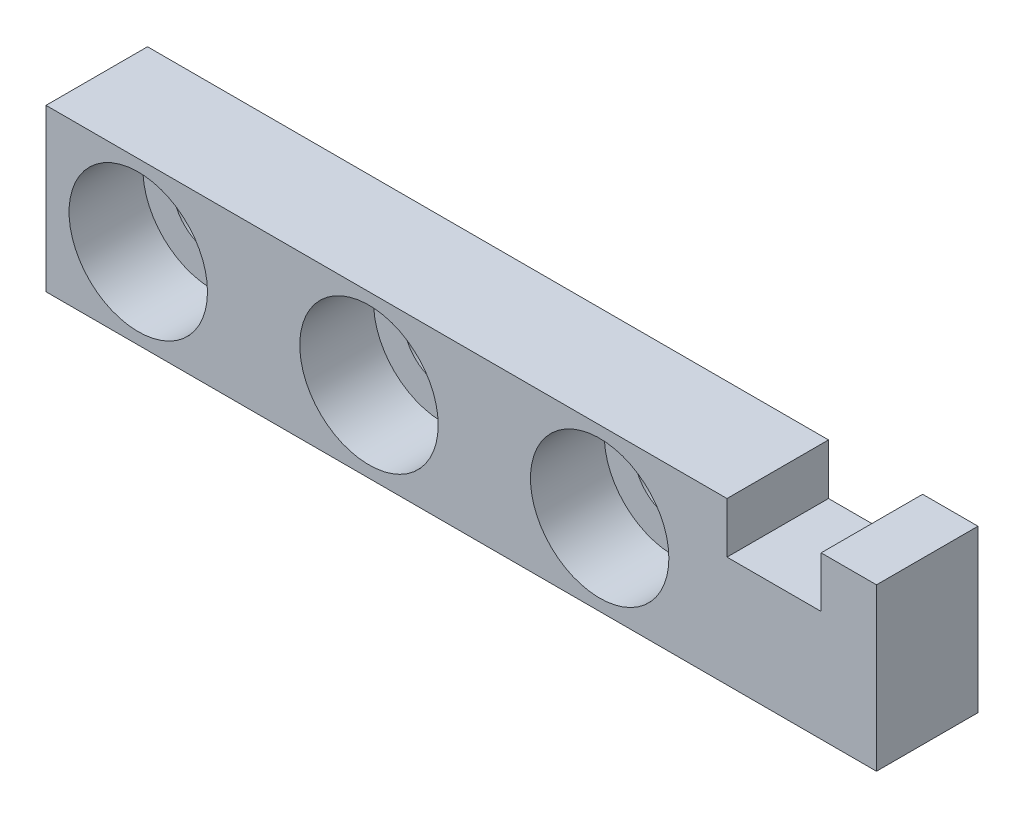
SolidWorks part; units mm, degrees
ref_plane "Front Plane" through (0, 0, 0) normal (0, 0, 1) x (1, 0, 0)
ref_plane "Top Plane" through (0, 0, 0) normal (0, 1, 0) x (1, 0, 0)
ref_plane "Right Plane" through (0, 0, 0) normal (1, 0, 0) x (0, 0, -1)
sketch "Sketch1" plane through (0, 0, 0) normal (0, 0, 1) x (1, 0, 0)
  line L0 (-45, 0) -> (45, 0) construction
  line L1 (-45, 8.75) -> (28.8, 8.75)
  line L2 (-45, 8.75) -> (-45, -8.75)
  line L3 (-45, -8.75) -> (45, -8.75)
  line L4 (45, 8.75) -> (45, -8.75)
  line L5 (-45, 8.75) -> (45, -8.75) construction
  line L6 (-45, -8.75) -> (45, 8.75) construction
  line L7 (28.8, 8.75) -> (28.8, 3.25)
  line L8 (28.8, 3.25) -> (39, 3.25)
  line L9 (39, 3.25) -> (39, 8.75)
  line L10 (39, 8.75) -> (45, 8.75)
  circle A0 centre (-35, 0) radius 4.25
  circle A1 centre (-10, 0) radius 4.25
  circle A2 centre (15, 0) radius 4.25
  point P0 (0, 0)
  dimension "D3" = 8.5
  dimension "D4" = 8.5
  dimension "D5" = 8.5
  dimension "D6" = 30
  dimension "D7" = 25
  dimension "D8" = 25
  dimension "D1" = 90
  dimension "D2" = 17.5
  dimension "D9" = 6
  dimension "D10" = 10.2
  dimension "D11" = 5.5
extrude "Boss-Extrude1" add sketch "Sketch1" along normal blind 11
sketch "Sketch2" plane through (0, 0, 11) normal (0, 0, 1) x (1, 0, 0)
  circle A0 centre (-35, 0) radius 7.5
  circle A1 centre (-10, 0) radius 7.5
  circle A2 centre (15, 0) radius 7.5
  dimension "D1" = 15
  dimension "D2" = 15
  dimension "D3" = 15
extrude "Cut-Extrude1" cut sketch "Sketch2" against normal blind 8
